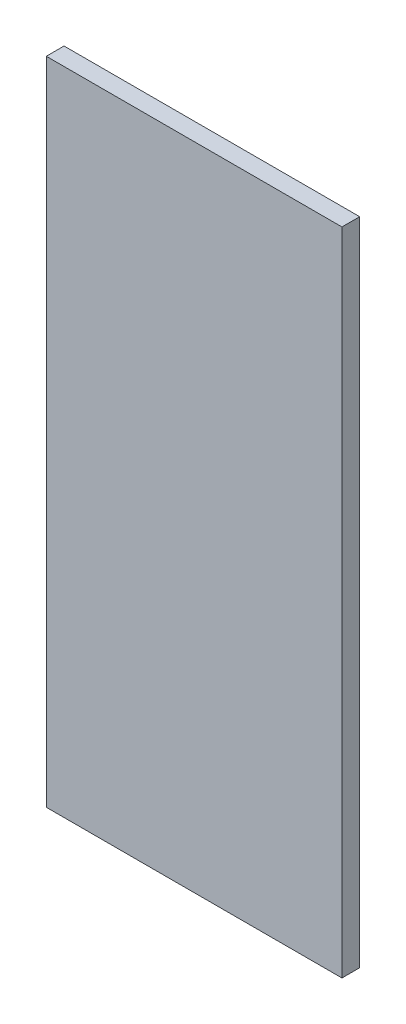
from build123d import *

# Parameters (mm, degrees)
SKETCH_1_W      = 100
SKETCH_1_H      = 220
EXTRUDE_1_DEPTH = 6


with BuildPart() as part:
    # 草图1 → 凸台-拉伸1 (new body)
    with BuildSketch(Plane.XY):
        Rectangle(SKETCH_1_W, SKETCH_1_H)
    extrude(amount=EXTRUDE_1_DEPTH)


solid = part.part
